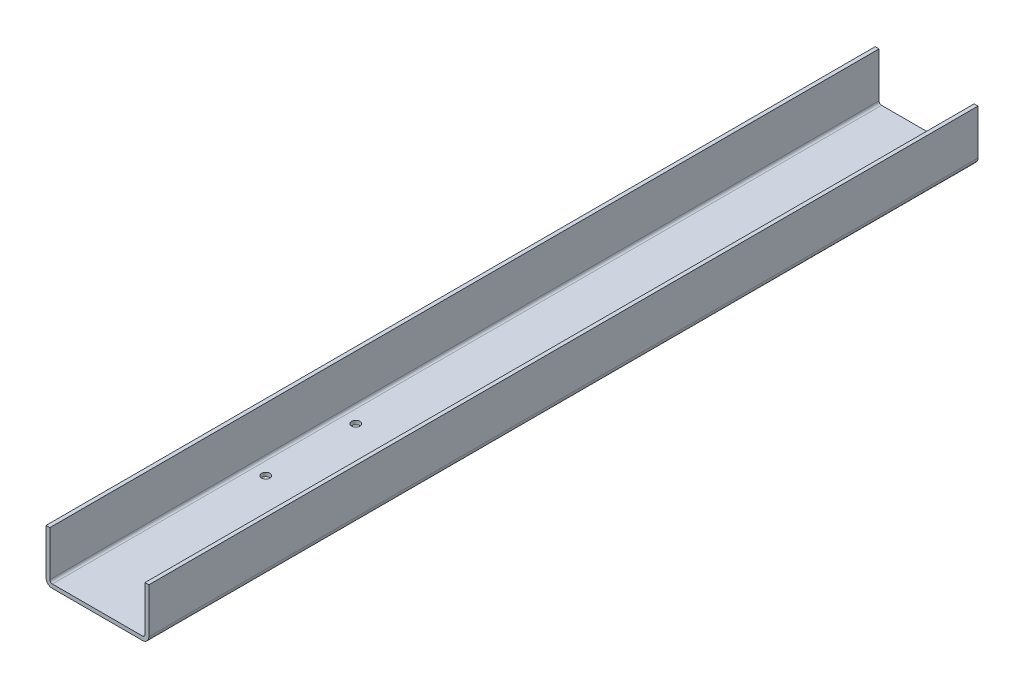
from build123d import *

# Parameters (mm, degrees)
BOSS_EXTRUDE1_DEPTH = 645
SKETCH2_R           = 3.25
CUT_EXTRUDE1_DEPTH  = 10


with BuildPart() as part:
    # Sketch1 → Boss-Extrude1 (new body)
    with BuildSketch(Plane.XY):
        with BuildLine():
            Line((0, 0), (0, -35))
            ThreePointArc((0, -35), (1.464466094, -38.535533906), (5, -40))
            Line((5, -40), (75, -40))
            ThreePointArc((75, -40), (78.535533906, -38.535533906), (80, -35))
            Line((80, -35), (80, 0))
            Line((80, 0), (77, 0))
            Line((77, 0), (77, -35))
            ThreePointArc((77, -35), (76.414213562, -36.414213562), (75, -37))
            Line((75, -37), (5, -37))
            ThreePointArc((5, -37), (3.585786438, -36.414213562), (3, -35))
            Line((3, -35), (3, 0))
            Line((3, 0), (0, 0))
        make_face()
    extrude(amount=BOSS_EXTRUDE1_DEPTH)

    # Sketch2 → Cut-Extrude1 (cut)
    with BuildSketch(Plane.XZ.offset(40)):
        with Locations(Location((15, 489, 0), (0, 0, 270))):
            Circle(SKETCH2_R)
        with Locations(Location((65, 489, 0), (0, 0, 270))):
            Circle(SKETCH2_R)
        with Locations(Location((15, 419, 0), (0, 0, 270))):
            Circle(SKETCH2_R)
        with Locations(Location((65, 419, 0), (0, 0, 270))):
            Circle(SKETCH2_R)
    extrude(amount=-CUT_EXTRUDE1_DEPTH, mode=Mode.SUBTRACT)


solid = part.part
